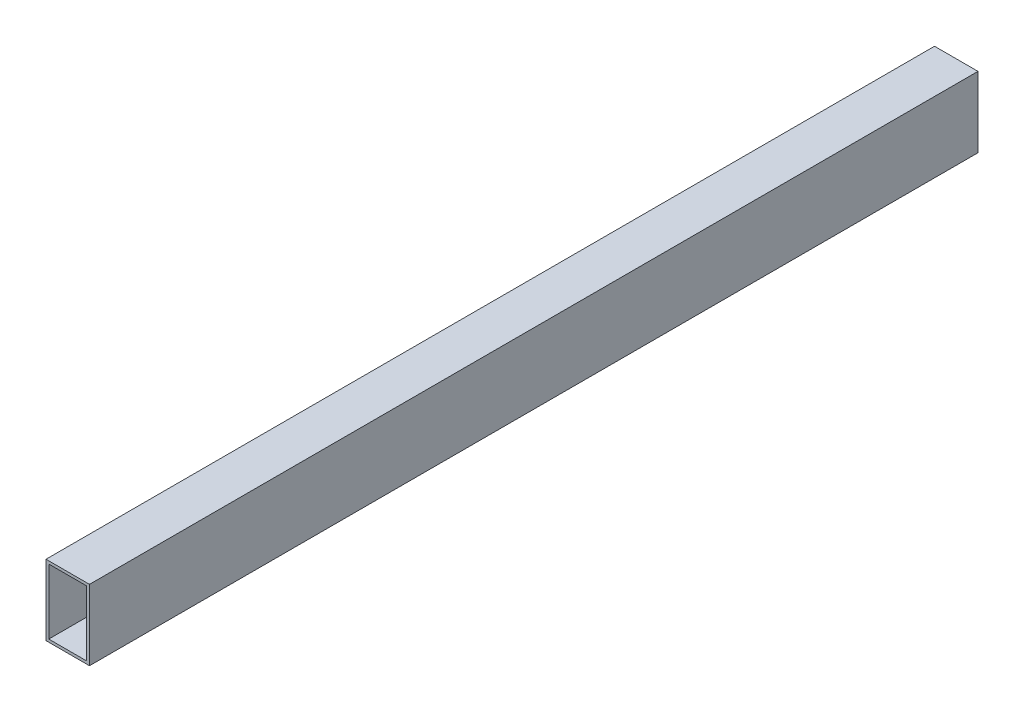
from build123d import *

# Parameters (mm, degrees)
SKETCH1_W           = 31.515629069
SKETCH1_H           = 51.109180057
SKETCH1_W_2         = 27.515629069
SKETCH1_H_2         = 47.109180057
BOSS_EXTRUDE1_DEPTH = 644


with BuildPart() as part:
    # Sketch1 → Boss-Extrude1 (new body)
    with BuildSketch(Plane.XY):
        with Locations((-64.747167395, 1.270489558)):
            Rectangle(SKETCH1_W, SKETCH1_H)
        with Locations((-64.747167395, 1.270489558)):
            Rectangle(SKETCH1_W_2, SKETCH1_H_2, mode=Mode.SUBTRACT)
    extrude(amount=BOSS_EXTRUDE1_DEPTH)


solid = part.part
